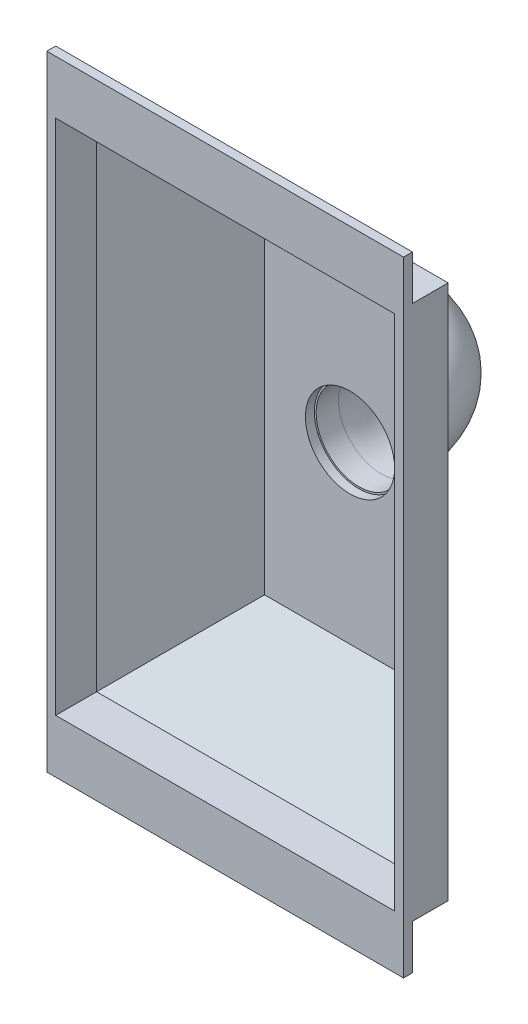
from build123d import *

# Parameters (mm, degrees)
SKETCH_1_W          = 400
SKETCH_1_H          = 600
EXTRUDE_1_DEPTH     = 150
CHAMFER_2_SIZE      = 100
SHELL_1_T           = -10
SKETCH_4_R          = 50
CUT_EXTRUDE_2_DEPTH = 387.781592116
SKETCH_6_R          = 50
SHELL_2_T           = -2
SKETCH_7_W          = 400
SKETCH_7_H          = 50
EXTRUDE_3_DEPTH     = 10


with BuildPart() as part:
    # 草图1 → 凸台-拉伸1 (new body)
    with BuildSketch(Plane.XY):
        Rectangle(SKETCH_1_W, SKETCH_1_H)
    extrude(amount=EXTRUDE_1_DEPTH)

    # 倒角2
    chamfer_2_edges = [part.edges().sort_by_distance(p)[0] for p in [
        (0, -300, 0),
        (-200, 0, 0),
        (0, 300, 0),
        (200, 0, 0),
    ]]
    chamfer(chamfer_2_edges, length=CHAMFER_2_SIZE)

    # 抽壳1
    shell_1_openings = [part.faces().sort_by_distance(p)[0] for p in [
        (0, 0, 150),
    ]]
    offset(amount=SHELL_1_T, openings=shell_1_openings, kind=Kind.INTERSECTION)

    # 草图4 → 切除-拉伸2 (cut, through all)
    with BuildSketch(Plane.XY.offset(10)):
        Circle(SKETCH_4_R)
    extrude(amount=-CUT_EXTRUDE_2_DEPTH, mode=Mode.SUBTRACT)

    # 草图7 → 凸台-拉伸3 (add)
    with BuildSketch(Plane.XY.offset(150)):
        with Locations((0, 325)):
            Rectangle(SKETCH_7_W, SKETCH_7_H)
        with Locations((0, -325)):
            Rectangle(SKETCH_7_W, SKETCH_7_H)
    extrude(amount=-EXTRUDE_3_DEPTH)


with BuildPart() as body_2:
    # 扫描1: sweep along a path in 草图5
    with BuildLine(Plane(origin=(0, 0, 0), x_dir=(1, 0, 0), z_dir=(0, 1, 0))) as sweep_1_path:
        Line((0, 0), (0, 25))
        ThreePointArc((0, 25), (-29.289321881, 95.710678119), (-100, 125))
        Line((-100, 125), (-300, 125))
    # 草图6 → 扫描1 (sweep)
    with BuildSketch(Plane(origin=(0, 0, 0), x_dir=(-1, 0, 0), z_dir=(0, 0, -1))):
        Circle(SKETCH_6_R)
    sweep(path=sweep_1_path.line)

    # 抽壳2
    shell_2_openings = [body_2.faces().sort_by_distance(p)[0] for p in [
        (-300, 0, -125),
        (0, 0, 0),
    ]]
    offset(amount=SHELL_2_T, openings=shell_2_openings, kind=Kind.INTERSECTION)


solid = Compound([part.part, body_2.part])
